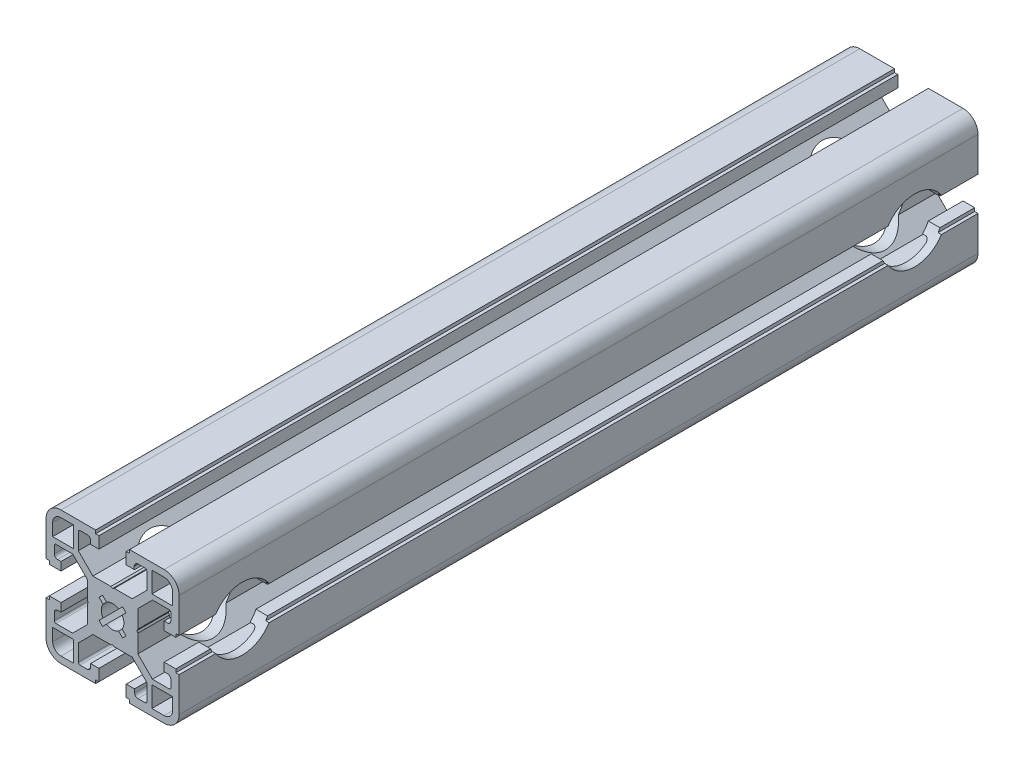
from build123d import *

# Parameters (mm, degrees)
EXTRUDE_1_DEPTH         = 240
HOLE_WIZARD_19_0_19_1_D = 19


with BuildPart() as part:
    # 草图1 → 凸台-拉伸1 (new body)
    with BuildSketch(Plane.XY):
        with BuildLine():
            Line((-18.9995, -4.100341675), (-18.9995, -5.100341675))
            Line((-18.9995, -5.100341675), (-19.9995, -5.100341675))
            Line((-19.9995, -5.100341675), (-19.9995, -15.500341675))
            ThreePointArc((-19.9995, -15.500341675), (-18.681480515, -18.682322191), (-15.4995, -20.000341675))
            Line((-15.4995, -20.000341675), (-5.0995, -20.000341675))
            Line((-5.0995, -20.000341675), (-5.0995, -19.000341675))
            Line((-5.0995, -19.000341675), (-4.0995, -19.000341675))
            Line((-4.0995, -19.000341675), (-4.0995, -15.500341675))
            Line((-4.0995, -15.500341675), (-6.5995, -15.500341675))
            Line((-6.5995, -15.500341675), (-6.5995, -16.500341675))
            ThreePointArc((-6.5995, -16.500341675), (-6.892393219, -17.207448457), (-7.5995, -17.500341675))
            Line((-7.5995, -17.500341675), (-9.7995, -17.500341675))
            ThreePointArc((-9.7995, -17.500341675), (-10.153053391, -17.353895066), (-10.2995, -17.000341675))
            Line((-10.2995, -17.000341675), (-10.2995, -11.997341675))
            Line((-10.2995, -11.997341675), (-5.9025, -7.600341675))
            Line((-5.9025, -7.600341675), (-0.5195, -7.600341675))
            Line((-0.5195, -7.600341675), (0.0005, -7.300341675))
            Line((0.0005, -7.300341675), (0.5195, -7.600341675))
            Line((0.5195, -7.600341675), (5.9035, -7.600341675))
            Line((5.9035, -7.600341675), (10.3005, -11.997341675))
            Line((10.3005, -11.997341675), (10.3005, -17.000341675))
            ThreePointArc((10.3005, -17.000341675), (10.154053391, -17.353895066), (9.8005, -17.500341675))
            Line((9.8005, -17.500341675), (7.6005, -17.500341675))
            ThreePointArc((7.6005, -17.500341675), (6.893393219, -17.207448457), (6.6005, -16.500341675))
            Line((6.6005, -16.500341675), (6.6005, -15.500341675))
            Line((6.6005, -15.500341675), (4.1005, -15.500341675))
            Line((4.1005, -15.500341675), (4.1005, -19.000341675))
            Line((4.1005, -19.000341675), (5.1005, -19.000341675))
            Line((5.1005, -19.000341675), (5.1005, -20.000341675))
            Line((5.1005, -20.000341675), (15.5005, -20.000341675))
            ThreePointArc((15.5005, -20.000341675), (18.682480515, -18.682322191), (20.0005, -15.500341675))
            Line((20.0005, -15.500341675), (20.0005, -5.100341675))
            Line((20.0005, -5.100341675), (19.0005, -5.100341675))
            Line((19.0005, -5.100341675), (19.0005, -4.100341675))
            Line((19.0005, -4.100341675), (15.5005, -4.100341675))
            Line((15.5005, -4.100341675), (15.5005, -6.600341675))
            Line((15.5005, -6.600341675), (16.5005, -6.600341675))
            ThreePointArc((16.5005, -6.600341675), (17.207606781, -6.893234894), (17.5005, -7.600341675))
            Line((17.5005, -7.600341675), (17.5005, -9.800341675))
            ThreePointArc((17.5005, -9.800341675), (17.354053391, -10.153895066), (17.0005, -10.300341675))
            Line((17.0005, -10.300341675), (11.9975, -10.300341675))
            Line((11.9975, -10.300341675), (7.6005, -5.903341675))
            Line((7.6005, -5.903341675), (7.6005, -0.520341675))
            Line((7.6005, -0.520341675), (7.3005, -0.000341675))
            Line((7.3005, -0.000341675), (7.6005, 0.519658325))
            Line((7.6005, 0.519658325), (7.6005, 5.902658325))
            Line((7.6005, 5.902658325), (11.9975, 10.299658325))
            Line((11.9975, 10.299658325), (17.0005, 10.299658325))
            ThreePointArc((17.0005, 10.299658325), (17.354053391, 10.153211715), (17.5005, 9.799658325))
            Line((17.5005, 9.799658325), (17.5005, 7.599658325))
            ThreePointArc((17.5005, 7.599658325), (17.207606781, 6.892551543), (16.5005, 6.599658325))
            Line((16.5005, 6.599658325), (15.5005, 6.599658325))
            Line((15.5005, 6.599658325), (15.5005, 4.099658325))
            Line((15.5005, 4.099658325), (19.0005, 4.099658325))
            Line((19.0005, 4.099658325), (19.0005, 5.099658325))
            Line((19.0005, 5.099658325), (20.0005, 5.099658325))
            Line((20.0005, 5.099658325), (20.0005, 15.499658325))
            ThreePointArc((20.0005, 15.499658325), (18.682480515, 18.68163884), (15.5005, 19.999658325))
            Line((15.5005, 19.999658325), (5.1005, 19.999658325))
            Line((5.1005, 19.999658325), (5.1005, 18.999658325))
            Line((5.1005, 18.999658325), (4.1005, 18.999658325))
            Line((4.1005, 18.999658325), (4.1005, 15.499658325))
            Line((4.1005, 15.499658325), (6.6005, 15.499658325))
            ThreePointArc((6.6005, 15.499658325), (6.393348977, 15.999658325), (6.6005, 16.499658325))
            ThreePointArc((6.6005, 16.499658325), (6.893393219, 17.206765106), (7.6005, 17.499658325))
            Line((7.6005, 17.499658325), (9.8005, 17.499658325))
            ThreePointArc((9.8005, 17.499658325), (10.154053391, 17.353211715), (10.3005, 16.999658325))
            Line((10.3005, 16.999658325), (10.3005, 11.996658325))
            Line((10.3005, 11.996658325), (5.9035, 7.599658325))
            Line((5.9035, 7.599658325), (0.5195, 7.599658325))
            Line((0.5195, 7.599658325), (0.0005, 7.299658325))
            Line((0.0005, 7.299658325), (-0.5195, 7.599658325))
            Line((-0.5195, 7.599658325), (-5.9025, 7.599658325))
            Line((-5.9025, 7.599658325), (-10.2995, 11.996658325))
            Line((-10.2995, 11.996658325), (-10.2995, 16.999658325))
            ThreePointArc((-10.2995, 16.999658325), (-10.153053391, 17.353211715), (-9.7995, 17.499658325))
            Line((-9.7995, 17.499658325), (-7.5995, 17.499658325))
            ThreePointArc((-7.5995, 17.499658325), (-6.892393219, 17.206765106), (-6.5995, 16.499658325))
            Line((-6.5995, 16.499658325), (-6.5995, 15.499658325))
            Line((-6.5995, 15.499658325), (-4.0995, 15.499658325))
            Line((-4.0995, 15.499658325), (-4.0995, 18.999658325))
            Line((-4.0995, 18.999658325), (-5.0995, 18.999658325))
            Line((-5.0995, 18.999658325), (-5.0995, 19.999658325))
            Line((-5.0995, 19.999658325), (-15.4995, 19.999658325))
            ThreePointArc((-15.4995, 19.999658325), (-18.681480515, 18.68163884), (-19.9995, 15.499658325))
            Line((-19.9995, 15.499658325), (-19.9995, 5.099658325))
            Line((-19.9995, 5.099658325), (-18.9995, 5.099658325))
            Line((-18.9995, 5.099658325), (-18.9995, 4.099658325))
            Line((-18.9995, 4.099658325), (-15.4995, 4.099658325))
            Line((-15.4995, 4.099658325), (-15.4995, 6.599658325))
            Line((-15.4995, 6.599658325), (-16.4995, 6.599658325))
            ThreePointArc((-16.4995, 6.599658325), (-17.206606781, 6.892551543), (-17.4995, 7.599658325))
            Line((-17.4995, 7.599658325), (-17.4995, 9.799658325))
            ThreePointArc((-17.4995, 9.799658325), (-17.353053391, 10.153211715), (-16.9995, 10.299658325))
            Line((-16.9995, 10.299658325), (-11.9965, 10.299658325))
            Line((-11.9965, 10.299658325), (-7.5995, 5.902658325))
            Line((-7.5995, 5.902658325), (-7.5995, 0.519658325))
            Line((-7.5995, 0.519658325), (-7.2995, -0.000341675))
            Line((-7.2995, -0.000341675), (-7.5995, -0.520341675))
            Line((-7.5995, -0.520341675), (-7.5995, -5.903341675))
            Line((-7.5995, -5.903341675), (-11.9965, -10.300341675))
            Line((-11.9965, -10.300341675), (-16.9995, -10.300341675))
            ThreePointArc((-16.9995, -10.300341675), (-17.353053391, -10.153895066), (-17.4995, -9.800341675))
            Line((-17.4995, -9.800341675), (-17.4995, -7.600341675))
            ThreePointArc((-17.4995, -7.600341675), (-17.206606781, -6.893234894), (-16.4995, -6.600341675))
            Line((-16.4995, -6.600341675), (-15.4995, -6.600341675))
            Line((-15.4995, -6.600341675), (-15.4995, -4.100341675))
            Line((-15.4995, -4.100341675), (-18.9995, -4.100341675))
        make_face()
        with BuildLine():
            Line((15.5005, -18.000341675), (11.8005, -18.000341675))
            Line((11.8005, -18.000341675), (11.8005, -11.800341675))
            Line((11.8005, -11.800341675), (18.0005, -11.800341675))
            Line((18.0005, -11.800341675), (18.0005, -15.500341675))
            ThreePointArc((18.0005, -15.500341675), (17.268266953, -17.268108628), (15.5005, -18.000341675))
        make_face(mode=Mode.SUBTRACT)
        with BuildLine():
            Line((18.0005, 11.799658325), (11.8005, 11.799658325))
            Line((11.8005, 11.799658325), (11.8005, 17.999658325))
            Line((11.8005, 17.999658325), (15.5005, 17.999658325))
            ThreePointArc((15.5005, 17.999658325), (17.268266953, 17.267425278), (18.0005, 15.499658325))
            Line((18.0005, 15.499658325), (18.0005, 11.799658325))
        make_face(mode=Mode.SUBTRACT)
        with BuildLine():
            Line((-1.8145, -2.875341675), (-3.004391671, -4.066450004))
            Line((-3.004391671, -4.066450004), (-4.065608329, -3.005233346))
            Line((-4.065608329, -3.005233346), (-2.8745, -1.815341675))
            ThreePointArc((-2.8745, -1.815341675), (-3.399473913, -0.000341675), (-2.8745, 1.814658325))
            Line((-2.8745, 1.814658325), (-4.064391671, 3.005766654))
            Line((-4.064391671, 3.005766654), (-3.004391671, 4.065766654))
            Line((-3.004391671, 4.065766654), (-1.8145, 2.874658325))
            ThreePointArc((-1.8145, 2.874658325), (0, 3.399316649), (1.8145, 2.874658325))
            Line((1.8145, 2.874658325), (3.0055, 4.065658325))
            Line((3.0055, 4.065658325), (4.066608329, 3.004549996))
            Line((4.066608329, 3.004549996), (2.8755, 1.814658325))
            ThreePointArc((2.8755, 1.814658325), (3.400473913, -0.000341675), (2.8755, -1.815341675))
            Line((2.8755, -1.815341675), (4.066608329, -3.005233346))
            Line((4.066608329, -3.005233346), (3.0055, -4.066341675))
            Line((3.0055, -4.066341675), (1.8145, -2.875341675))
            ThreePointArc((1.8145, -2.875341675), (0, -3.4), (-1.8145, -2.875341675))
        make_face(mode=Mode.SUBTRACT)
        with BuildLine():
            Line((-17.9995, -15.500341675), (-17.9995, -11.800341675))
            Line((-17.9995, -11.800341675), (-11.7995, -11.800341675))
            Line((-11.7995, -11.800341675), (-11.7995, -18.000341675))
            Line((-11.7995, -18.000341675), (-15.4995, -18.000341675))
            ThreePointArc((-15.4995, -18.000341675), (-17.267266953, -17.268108628), (-17.9995, -15.500341675))
        make_face(mode=Mode.SUBTRACT)
        with BuildLine():
            Line((-11.7995, 17.999658325), (-11.7995, 11.799658325))
            Line((-11.7995, 11.799658325), (-17.9995, 11.799658325))
            Line((-17.9995, 11.799658325), (-17.9995, 15.499658325))
            ThreePointArc((-17.9995, 15.499658325), (-17.267266953, 17.267425278), (-15.4995, 17.999658325))
            Line((-15.4995, 17.999658325), (-11.7995, 17.999658325))
        make_face(mode=Mode.SUBTRACT)
    extrude(amount=-EXTRUDE_1_DEPTH)

    # Ø19.0 (19) 直径孔1 (through all)
    with Locations(Plane(origin=(20.0005, 0, 0), x_dir=(0, 0, -1), z_dir=(1, 0, 0))):
        with Locations((19, -0.000341675), (221, -0.000341675)):
            Hole(HOLE_WIZARD_19_0_19_1_D / 2)


solid = part.part
